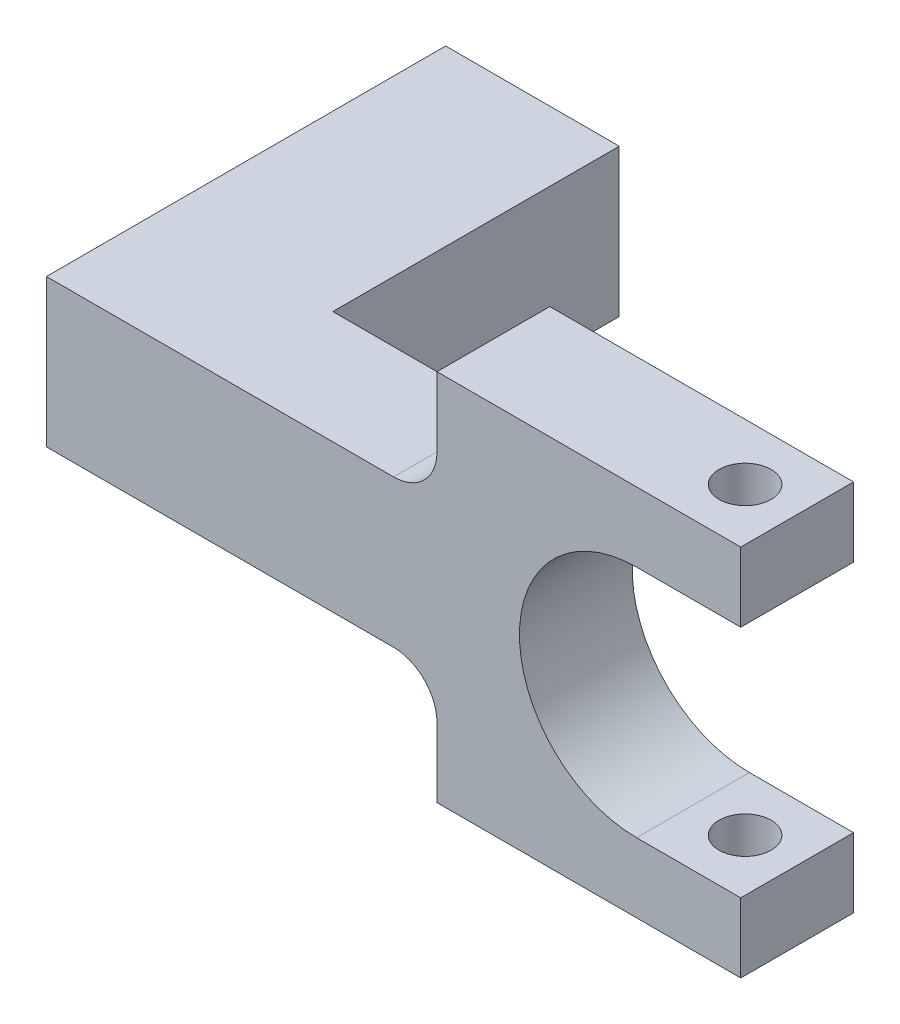
from build123d import *

# Parameters (mm, degrees)
EXTRUDE_1_DEPTH     = 6.5
CUT_EXTRUDE_1_REACH = 74.493
SKETCH_2_W          = 45
SKETCH_2_H          = 13
FILLET_1_R          = 5
SKETCH_3_W          = 20
SKETCH_3_H          = 17
EXTRUDE_2_DEPTH     = 33
CUT_EXTRUDE_2_REACH = 91.628
SKETCH_4_R          = 3


with BuildPart() as part:
    # 草图1 → 凸台-拉伸1 (new, symmetric)
    with BuildSketch(Plane.XY):
        with BuildLine():
            Line((0, 13.5), (12, 13.5))
            Line((12, 13.5), (12, 21.5))
            Line((12, 21.5), (-68, 21.5))
            Line((-68, 21.5), (-68, -21.5))
            Line((-68, -21.5), (12, -21.5))
            Line((12, -21.5), (12, -13.5))
            Line((12, -13.5), (0, -13.5))
            ThreePointArc((0, -13.5), (-13.5, 0), (0, 13.5))
        make_face()
    extrude(amount=EXTRUDE_1_DEPTH, both=True)

    # 草图2 → 切除-拉伸1 (cut, up to next)
    with BuildSketch(Plane.XY.offset(6.5), mode=Mode.PRIVATE) as cut_extrude_1_sk1:
        with Locations((-45.5, 15)):
            Rectangle(SKETCH_2_W, SKETCH_2_H)
    cut_extrude_1_tool1 = extrude(cut_extrude_1_sk1.sketch, amount=-CUT_EXTRUDE_1_REACH, mode=Mode.PRIVATE) & part.part
    # 草图2 → 切除-拉伸1 (cut, up to next)
    with BuildSketch(Plane.XY.offset(6.5), mode=Mode.PRIVATE) as cut_extrude_1_sk2:
        with Locations((-45.5, -15)):
            Rectangle(SKETCH_2_W, SKETCH_2_H)
    cut_extrude_1_tool2 = extrude(cut_extrude_1_sk2.sketch, amount=-CUT_EXTRUDE_1_REACH, mode=Mode.PRIVATE) & part.part
    add(cut_extrude_1_tool1.solids().sort_by_distance((-45.5, 15, 6.5))[0], mode=Mode.SUBTRACT)
    add(cut_extrude_1_tool2.solids().sort_by_distance((-45.5, -15, 6.5))[0], mode=Mode.SUBTRACT)

    # 圆角1
    fillet_1_edges = [part.edges().sort_by_distance(p)[0] for p in [
        (-23, 8.5, 0),
        (-23, -8.5, 0),
    ]]
    fillet(fillet_1_edges, radius=FILLET_1_R)

    # 草图3 → 凸台-拉伸2 (add)
    with BuildSketch(Plane(origin=(0, 0, -6.5), x_dir=(-1, 0, 0), z_dir=(0, 0, -1))):
        with Locations((58, 0)):
            Rectangle(SKETCH_3_W, SKETCH_3_H)
    extrude(amount=EXTRUDE_2_DEPTH)

    # 切除-拉伸2: up to this face of the body (flat: up to its plane)
    cut_extrude_2_end = Plane(part.part.faces().sort_by_distance((-5.5, 21.5, 0))[0])
    # 草图4 → 切除-拉伸2 (cut, up to the picked face)
    with BuildSketch(Plane.XZ.offset(21.5), mode=Mode.PRIVATE) as cut_extrude_2_sk1:
        with Locations(Location((6, 0, 0), (0, 0, 270))):
            Circle(SKETCH_4_R)
    cut_extrude_2_tool1 = split(extrude(cut_extrude_2_sk1.sketch, amount=-CUT_EXTRUDE_2_REACH, mode=Mode.PRIVATE), bisect_by=cut_extrude_2_end, keep=Keep.BOTH, mode=Mode.PRIVATE)
    add(cut_extrude_2_tool1.solids().sort_by(Axis((6, -21.5, 0), (0, 1, 0)))[0], mode=Mode.SUBTRACT)


solid = part.part
